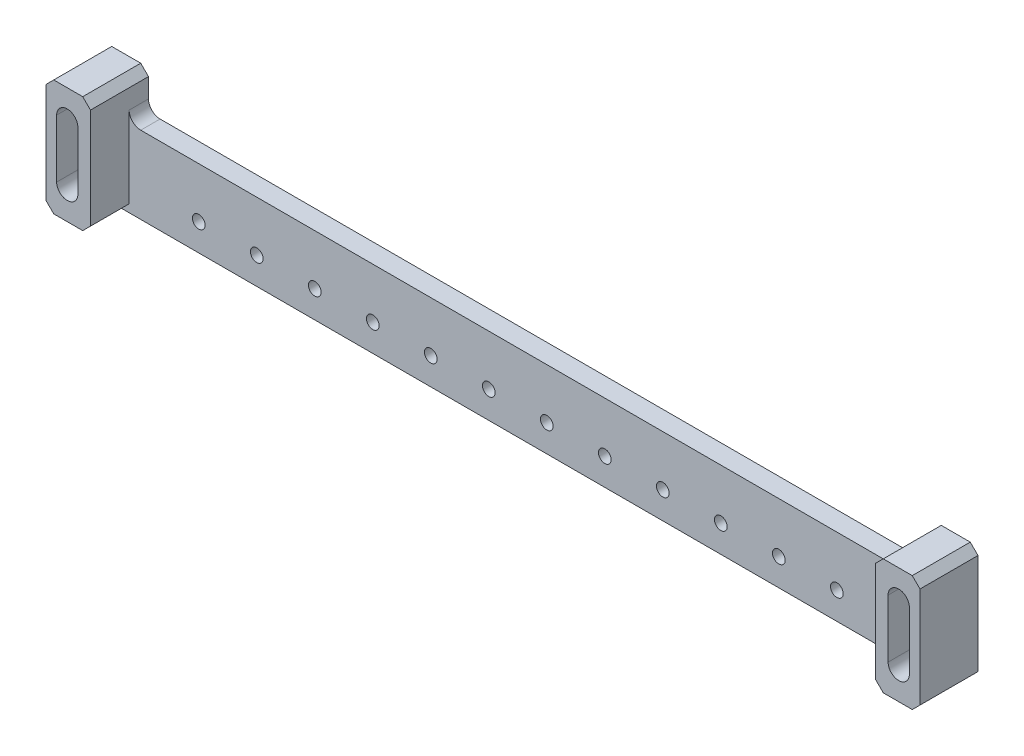
from build123d import *

# Parameters (mm, degrees)
SKETCH_1_W             = 226
SKETCH_1_H             = 30
EXTRUDE_1_DEPTH        = 15
SKETCH_2_W             = 203
SKETCH_2_H             = 30
CUT_EXTRUDE_1_DEPTH    = 10
SKETCH_3_W             = 203
SKETCH_3_H             = 10
CUT_EXTRUDE_2_DEPTH    = 115.429017299
CUT_EXTRUDE_3_DEPTH    = 115.973910084
CUT_EXTRUDE_4_DEPTH    = 6
HOLE_WIZARD_M4_1_D     = 3.3
PATTERN_LINEAR_1_COUNT = 12
PATTERN_LINEAR_1_PITCH = 15
CHAMFER_1_SIZE         = 2
FILLET_1_R             = 3


with BuildPart() as part:
    # 草图1 → 凸台-拉伸1 (new body)
    with BuildSketch(Plane.XY):
        Rectangle(SKETCH_1_W, SKETCH_1_H)
    extrude(amount=EXTRUDE_1_DEPTH)

    # 草图2 → 切除-拉伸1 (cut)
    with BuildSketch(Plane.XY.offset(15)):
        Rectangle(SKETCH_2_W, SKETCH_2_H)
    extrude(amount=-CUT_EXTRUDE_1_DEPTH, mode=Mode.SUBTRACT)

    # 草图3 → 切除-拉伸2 (cut, through all)
    with BuildSketch(Plane.XY.offset(5)):
        with Locations((0, 10)):
            Rectangle(SKETCH_3_W, SKETCH_3_H)
    extrude(amount=-CUT_EXTRUDE_2_DEPTH, mode=Mode.SUBTRACT)

    # 草图4 → 切除-拉伸3 (cut, through all)
    with BuildSketch(Plane(origin=(0, 0, 0), x_dir=(-1, 0, 0), z_dir=(0, 0, -1))):
        with BuildLine():
            Line((104.75, -7.5), (104.75, 7.5))
            ThreePointArc((104.75, 7.5), (107.5, 10.25), (110.25, 7.5))
            Line((110.25, 7.5), (110.25, -7.5))
            ThreePointArc((110.25, -7.5), (107.5, -10.25), (104.75, -7.5))
        make_face()
        with BuildLine():
            Line((-110.25, -7.5), (-110.25, 7.5))
            ThreePointArc((-110.25, 7.5), (-107.5, 10.25), (-104.75, 7.5))
            Line((-104.75, 7.5), (-104.75, -7.5))
            ThreePointArc((-104.75, -7.5), (-107.5, -10.25), (-110.25, -7.5))
        make_face()
    extrude(amount=-CUT_EXTRUDE_3_DEPTH, mode=Mode.SUBTRACT)

    # 草图5 → 切除-拉伸4 (cut)
    with BuildSketch(Plane(origin=(0, 0, 0), x_dir=(-1, 0, 0), z_dir=(0, 0, -1))):
        with BuildLine():
            Line((102.5, -7.5), (102.5, 7.5))
            ThreePointArc((102.5, 7.5), (107.5, 12.5), (112.5, 7.5))
            Line((112.5, 7.5), (112.5, -7.5))
            ThreePointArc((112.5, -7.5), (107.5, -12.5), (102.5, -7.5))
        make_face()
        with BuildLine():
            Line((-112.5, -7.5), (-112.5, 7.5))
            ThreePointArc((-112.5, 7.5), (-107.5, 12.5), (-102.5, 7.5))
            Line((-102.5, 7.5), (-102.5, -7.5))
            ThreePointArc((-102.5, -7.5), (-107.5, -12.5), (-112.5, -7.5))
        make_face()
    extrude(amount=-CUT_EXTRUDE_4_DEPTH, mode=Mode.SUBTRACT)

    # M4 螺纹孔1 (through all)
    with Locations(Plane(origin=(0, 0, 0), x_dir=(-1, 0, 0), z_dir=(0, 0, -1))):
        with Locations((-81.5, -8)):
            hole_wizard_m4_1 = Hole(HOLE_WIZARD_M4_1_D / 2)

    # 阵列(线性)1: M4 螺纹孔1 ×12
    with Locations(*[(-i * PATTERN_LINEAR_1_PITCH, 0, 0) for i in range(1, PATTERN_LINEAR_1_COUNT)]):
        add(hole_wizard_m4_1, mode=Mode.SUBTRACT)

    # 倒角1
    chamfer_1_edges = [part.edges().sort_by_distance(p)[0] for p in [
        (101.5, 15, 7.5),
        (101.5, -15, 10),
        (-101.5, -15, 10),
        (-101.5, 15, 7.5),
        (113, -15, 7.5),
        (-113, -15, 7.5),
        (-113, 15, 7.5),
        (113, 15, 7.5),
    ]]
    chamfer(chamfer_1_edges, length=CHAMFER_1_SIZE)

    # 圆角1
    fillet_1_edges = [part.edges().sort_by_distance(p)[0] for p in [
        (-101.5, 5, 2.5),
        (101.5, 5, 2.5),
    ]]
    fillet(fillet_1_edges, radius=FILLET_1_R)


solid = part.part
